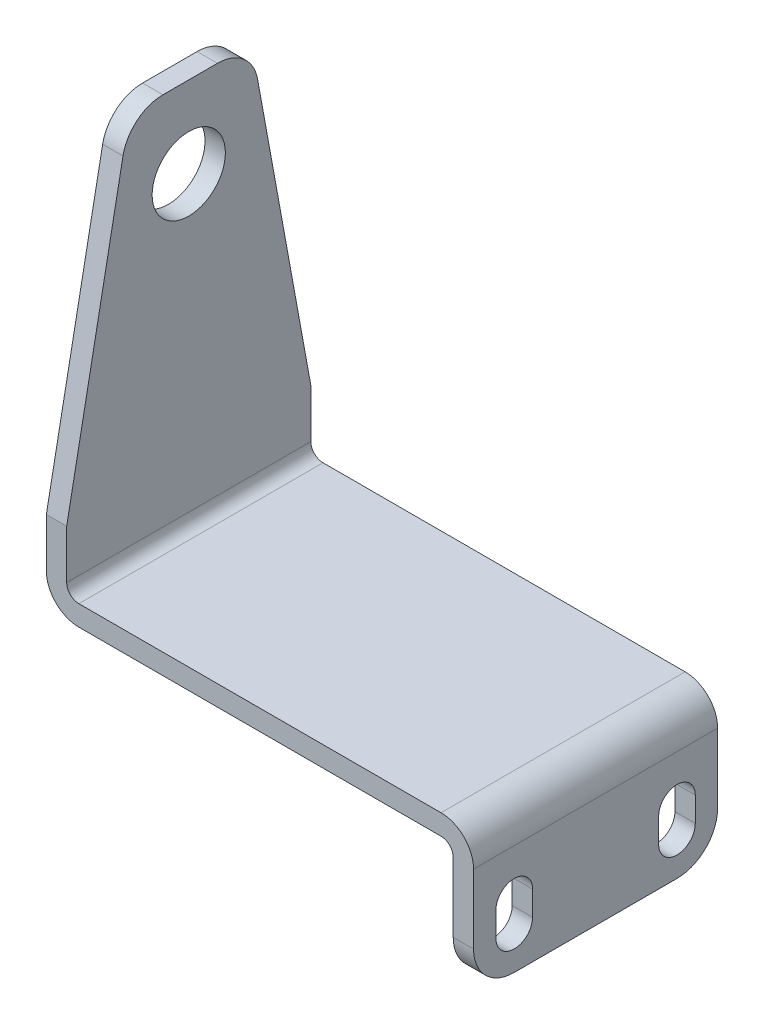
from build123d import *

# Parameters (mm, degrees)
BOSS_EXTRUDE1_DEPTH            = 5
SKETCH2_W                      = 60
SKETCH2_H                      = 35
BOSS_EXTRUDE2_DEPTH            = 100
SKETCH3_W                      = 100
SKETCH3_H                      = 30
CUT_EXTRUDE1_DEPTH             = 175.642491966
CUT_EXTRUDE2_DEPTH             = 175.642491966
CUT_EXTRUDE3_DEPTH             = 178.552809046
F_18_0_18_DIAMETER_HOLE1_D     = 18
F_18_0_18_DIAMETER_HOLE1_DEPTH = 105
FILLET1_R                      = 3
FILLET2_R                      = 8
FILLET3_R                      = 10


with BuildPart() as part:
    # Sketch1 → Boss-Extrude1 (new body)
    with BuildSketch(Plane(origin=(0, 0, 0), x_dir=(0, 0, -1), z_dir=(1, 0, 0))):
        Polygon((0, -80), (-14.600649986, 0), (-44.600649986, 0), (-60, -80), (-60, -130), (0, -130), align=None)
    extrude(amount=-BOSS_EXTRUDE1_DEPTH)

    # Sketch2 → Boss-Extrude2 (add)
    with BuildSketch(Plane(origin=(0, 0, 0), x_dir=(0, 0, -1), z_dir=(1, 0, 0))):
        with Locations((-30, -112.5)):
            Rectangle(SKETCH2_W, SKETCH2_H)
    extrude(amount=BOSS_EXTRUDE2_DEPTH)

    # Sketch3 → Cut-Extrude1 (cut, through all)
    with BuildSketch(Plane(origin=(0, 0, 0), x_dir=(-1, 0, 0), z_dir=(0, 0, -1))):
        with Locations((-45, -115)):
            Rectangle(SKETCH3_W, SKETCH3_H)
    extrude(amount=-CUT_EXTRUDE1_DEPTH, mode=Mode.SUBTRACT)

    # Sketch4 → Cut-Extrude2 (cut, through all)
    with BuildSketch(Plane.ZY.offset(-95)):
        with BuildLine():
            Line((54.5, -120.5), (54.5, -114.5))
            ThreePointArc((54.5, -114.5), (50, -110), (45.5, -114.5))
            Line((45.5, -114.5), (45.5, -120.5))
            ThreePointArc((45.5, -120.5), (50, -125), (54.5, -120.5))
        make_face()
    extrude(amount=-CUT_EXTRUDE2_DEPTH, mode=Mode.SUBTRACT)

    # Sketch5 → Cut-Extrude3 (cut, through all)
    with BuildSketch(Plane(origin=(100, 0, 0), x_dir=(0, 0, -1), z_dir=(1, 0, 0))):
        with BuildLine():
            Line((-14.5, -114.5), (-14.5, -120.5))
            ThreePointArc((-14.5, -120.5), (-10, -125), (-5.5, -120.5))
            Line((-5.5, -120.5), (-5.5, -114.5))
            ThreePointArc((-5.5, -114.5), (-10, -110), (-14.5, -114.5))
        make_face()
    extrude(amount=-CUT_EXTRUDE3_DEPTH, mode=Mode.SUBTRACT)

    # Ø18.0 (18) Diameter Hole1
    with Locations(Plane.ZY.offset(5)):
        with Locations((30, -20)):
            Hole(F_18_0_18_DIAMETER_HOLE1_D / 2, depth=F_18_0_18_DIAMETER_HOLE1_DEPTH)

    # Fillet1
    fillet1_edges = [part.edges().sort_by_distance(p)[0] for p in [
        (0, -95, 30),
        (95, -100, 30),
    ]]
    fillet(fillet1_edges, radius=FILLET1_R)

    # Fillet2
    fillet2_edges = [part.edges().sort_by_distance(p)[0] for p in [
        (100, -95, 30),
        (-5, -100, 30),
    ]]
    fillet(fillet2_edges, radius=FILLET2_R)

    # Fillet3
    fillet3_edges = [part.edges().sort_by_distance(p)[0] for p in [
        (-2.5, 0, 44.600649986),
        (-2.5, 0, 14.600649986),
        (97.5, -130, 60),
        (97.5, -130, 0),
    ]]
    fillet(fillet3_edges, radius=FILLET3_R)


solid = part.part
